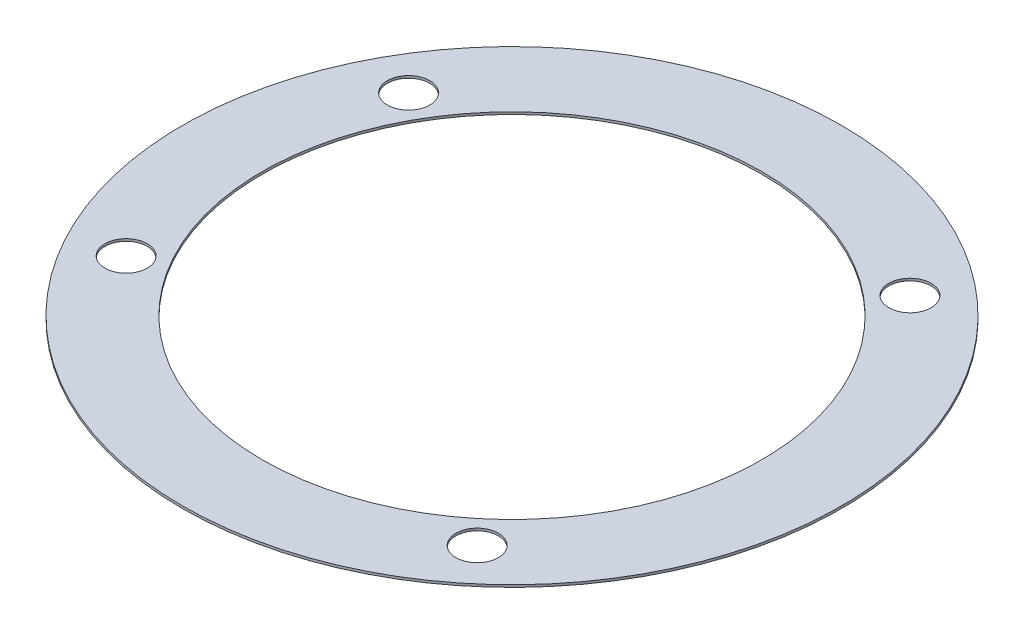
SolidWorks part; units mm, degrees
material "瓦楞纸"
ref_plane "Front Plane" through (0, 0, 0) normal (0, 0, 1) x (1, 0, 0)
ref_plane "Top Plane" through (0, 0, 0) normal (0, 1, 0) x (1, 0, 0)
ref_plane "Right Plane" through (0, 0, 0) normal (1, 0, 0) x (0, 0, -1)
sketch "Sketch1" plane through (0, 0, 0) normal (0, 1, 0) x (1, 0, 0)
  circle A0 centre (0, 0) radius 111.125
  circle A1 centre (0, 0) radius 84.2
  dimension "D1" = 222.25
  dimension "D2" = 168.4
extrude "Boss-Extrude1" add sketch "Sketch1" along normal blind 0.7937
hole_wizard "9/16 (0.5625) Diameter Hole1" positions "3DSketch1" profile "Sketch2" hole size "9/16" standard "Ansi Inch" end condition through all
sketch3d "3DSketch1"
  point P0 (61.2154, 0.7937, -72.9742)
  dimension "D1" = 72.9742
  dimension "D2" = 61.2154
sketch "Sketch2" plane through (61.2154, 0.7937, -72.9742) normal (1, 0, 0) x (0, 0, 1)
  line L0 (0, 0) -> (0, 0.7937)
  line L1 (0, 0.7937) -> (7.1437, 0.7937)
  line L2 (7.1437, 0.7937) -> (7.1437, 0)
  line L5 (7.1437, 0) -> (0, 0)
  line L11 (0, -6.35) -> (0, 107.95) construction
  dimension "通孔孔直径" = 14.2875
  dimension "通孔孔深度" = 0.7937
hole_wizard "9/16 (0.5625) Diameter Hole2" positions "Sketch4" profile "Sketch3" hole size "9/16" standard "Ansi Inch" end condition through all
sketch "Sketch4" plane through (0, 0, 0) normal (0, -1, 0) x (-1, 0, 0)
  line L0 (-0.4366, 0) -> (0.4366, 0) construction
  line L1 (0, 0.4366) -> (0, -0.4366) construction
  point P0 (82.4992, 47.625)
  dimension "D1" = 47.625
  dimension "D2" = 82.4992
sketch "Sketch3" plane through (-82.4992, 0, -47.625) normal (1, 0, 0) x (0, 0, -1)
  line L0 (0, 0) -> (0, 0.7937)
  line L1 (0, 0.7937) -> (7.1437, 0.7937)
  line L2 (7.1437, 0.7937) -> (7.1437, 0)
  line L5 (7.1437, 0) -> (0, 0)
  line L11 (0, -6.35) -> (0, 107.95) construction
  dimension "通孔孔直径" = 14.2875
  dimension "通孔孔深度" = 0.7938
mirror "Mirror1" about plane through (0, 0, 0) normal (0, 0, 1) of "9/16 (0.5625) Diameter Hole1", "9/16 (0.5625) Diameter Hole2"
